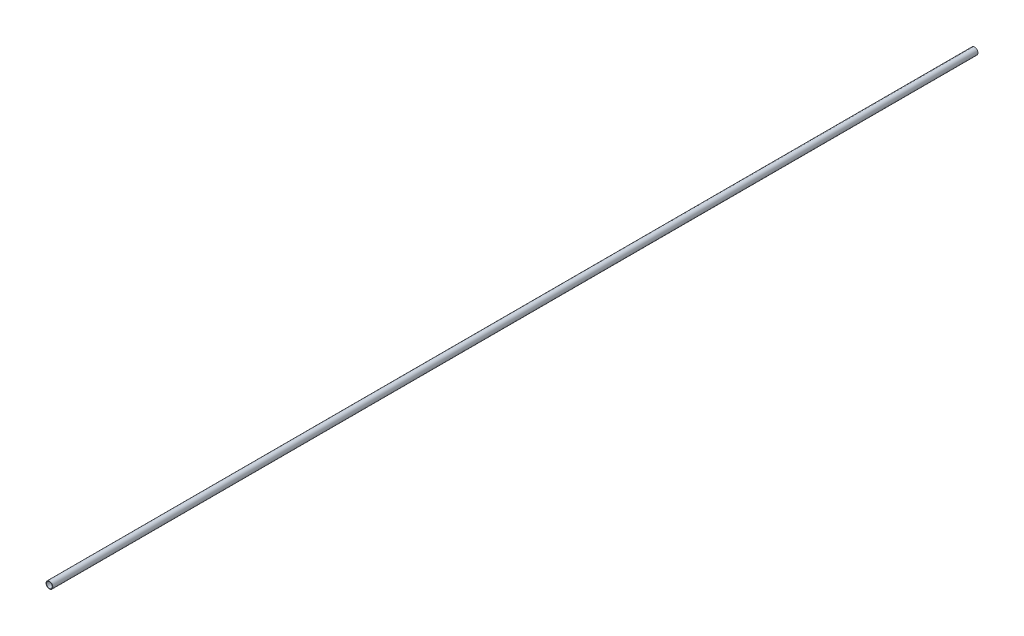
SolidWorks part; units mm, degrees
ref_plane "前视基准面" through (0, 0, 0) normal (0, 0, 1) x (1, 0, 0)
ref_plane "上视基准面" through (0, 0, 0) normal (0, 1, 0) x (1, 0, 0)
ref_plane "右视基准面" through (0, 0, 0) normal (1, 0, 0) x (0, 0, -1)
sketch "草图1" plane through (0, 0, 0) normal (0, 0, 1) x (1, 0, 0)
  circle A0 centre (0, 0) radius 12.5
  circle A1 centre (0, 0) radius 10.5
  dimension "D1" = 25
  dimension "D2" = 2
extrude "凸台-拉伸1" add sketch "草图1" along normal mid plane 3400
